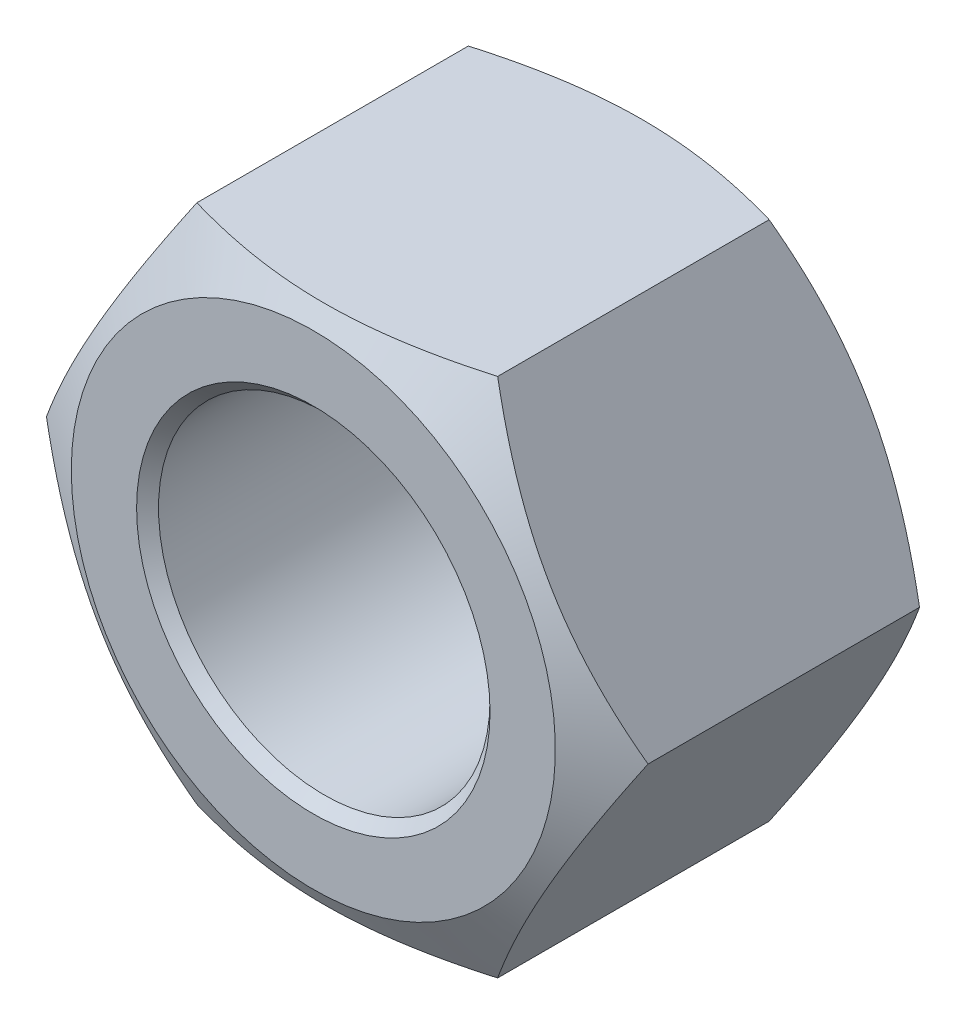
SolidWorks part; units mm, degrees
ref_plane "Front" through (0, 0, 0) normal (0, 0, 1) x (1, 0, 0)
ref_plane "Top" through (0, 0, 0) normal (0, 1, 0) x (1, 0, 0)
ref_plane "Right" through (0, 0, 0) normal (1, 0, 0) x (0, 0, -1)
other "Configuration Table"
sketch "Sketch1" plane through (0, 0, 0) normal (0, 0, 1) x (1, 0, 0)
  line L1 (15.8771, -27.5) -> (31.7543, 0)
  line L2 (31.7543, 0) -> (15.8771, 27.5)
  line L3 (15.8771, 27.5) -> (-15.8771, 27.5)
  line L4 (-15.8771, 27.5) -> (-31.7543, 0)
  line L5 (-31.7543, 0) -> (-15.8771, -27.5)
  line L6 (-15.8771, -27.5) -> (15.8771, -27.5)
  circle A0 centre (0, 0) radius 27.5 construction
  circle A1 centre (0, 0) radius 17.5
extrude "BaseNut" add sketch "Sketch1" against normal blind 34.7
cosmetic thread "ThreadCosmetic1" [suppressed] parameters "D2"=37
sketch "Sketch2" plane through (15.0481, 0, -16.7061) normal (0, 1, 0) x (0, 0, -1)
  line L0 (-23.7227, 15.0481) -> (22.0646, 15.0481) construction
  line L2 (17.9939, 46.8024) -> (17.9939, 30.9252) construction
  line L4 (17.9939, 46.8024) -> (-16.7061, 46.8024) construction
  line L8 (15.5376, 46.8024) -> (17.9939, 42.5481)
  line L9 (17.9939, 46.8024) -> (15.5376, 46.8024)
  line L10 (17.9939, 42.5481) -> (17.9939, 46.8024)
revolve "Chamfer1" cut sketch "Sketch2" angle 360 about L0
sketch "Sketch6" plane through (-9.1975, 0, -10.2525) normal (0, 1, 0) x (0, 0, 1)
  line L0 (23.3574, 9.1975) -> (-22.3023, 9.1975) construction
  line L2 (-24.4475, 26.6975) -> (-24.4475, 28.6475)
  line L4 (-24.4475, 28.6475) -> (-23.3216, 26.6975)
  line L6 (-23.3216, 26.6975) -> (-24.4475, 26.6975)
  dimension "da" = 38.9
  dimension "D2" = 60
revolve "EndChamfer1" cut sketch "Sketch6" angle 360 about L0
sketch "Sketch5" plane through (-14.793, 0, -16.9612) normal (0, 1, 0) x (0, 0, 1)
  line L0 (-22.5748, 14.793) -> (24.743, 14.793) construction
  line L2 (16.9612, 40.343) -> (16.9612, 46.5473)
  line L4 (16.9612, 46.5473) -> (13.3792, 46.5473)
  line L6 (13.3792, 46.5473) -> (16.9612, 40.343)
  dimension "dw1" = 51.1
  dimension "D2" = 30
revolve "Chamfer2" cut sketch "Sketch5" angle 360 about L0
sketch "Sketch3" plane through (-20.9491, 1.8856, 0) normal (0, 0, 1) x (1, 0, 0)
  circle A1 centre (20.9491, -1.8856) radius 17.5 construction
  circle A2 centre (20.9491, -1.8856) radius 25.55
  circle A3 centre (20.9491, -1.8856) radius 17.5
  dimension "dw" = 51.1
extrude "Extrude1" [suppressed] add sketch "Sketch3" along normal blind 0.8
chamfer "EndChamfer3" [suppressed] distance 1.1567 angle 45
chamfer "EndChamfer2" distance 1.1567 angle 45 1 edges at (17.5, 0, 0)
sketch "Sketch7" plane through (0, 0, 0) normal (0, 1, 0) x (1, 0, 0)
  line L0 (0, 48.6183) -> (0, -13.0076) construction
  line L1 (16.5, 34.0742) -> (17.5, 34.0742)
  line L2 (17.5, 34.0742) -> (18.366, 33.5742)
  line L3 (18.366, 33.5742) -> (17.5, 33.0742)
  line L4 (17.5, 33.0742) -> (16.5, 33.0742)
  line L5 (16.5, 33.0742) -> (16.5, 34.0742)
  line L6 (17.5, 33.5742) -> (-17.5, 33.5742) construction
revolve "Cut-Revolve10" [suppressed] cut sketch "Sketch7" angle 360 about L0
pattern_linear "LPattern10" [suppressed] count 28 spacing 1.2 along (0, 0, -1)
equation "\"D1@EndChamfer3\" = \"m@BaseNut\" / 30"
equation "\"D1@EndChamfer2\" = \"m@BaseNut\" / 30"
equation "\"s1@Sketch2\" = \"s@Sketch1\""
equation "\"D2@Sketch7\" = \"D1@Sketch1\""
equation "\"D1@Sketch7\" = (  \"D2@ThreadCosmetic1\" - \"D1@Sketch1\" )  / 2"
equation "\"D3@LPattern10\" = \"D1@Sketch7\" * 1.2"
equation "\"D1@LPattern10\" = \"m@BaseNut\" / \"D3@LPattern10\" - 1"
